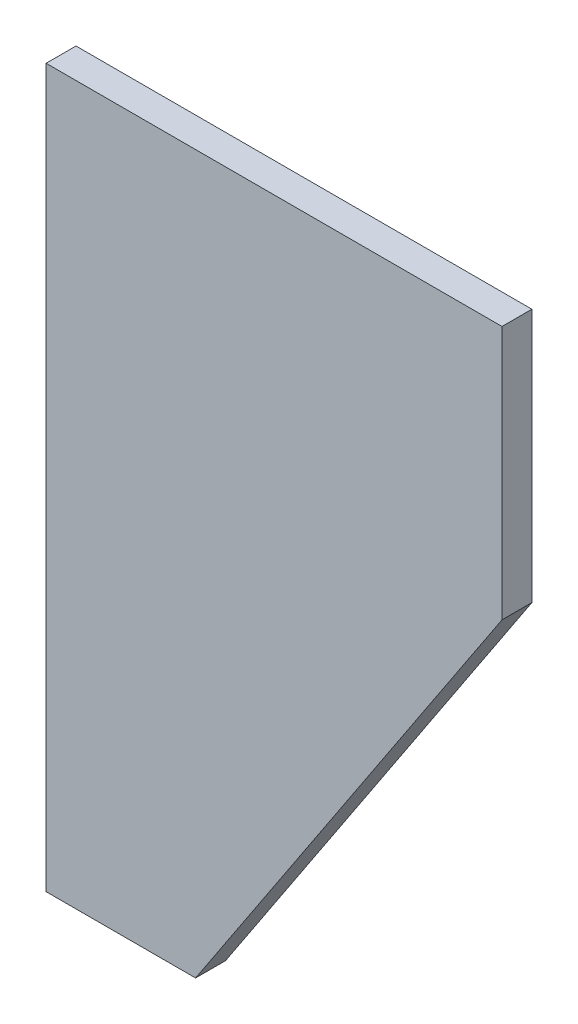
from build123d import *

# Parameters (mm, degrees)
EXTRUDE_1_DEPTH = 2


with BuildPart() as part:
    # 草图1 → 凸台-拉伸1 (new body)
    with BuildSketch(Plane.XY):
        Polygon((0, 0), (30.5, 0), (30.5, -17), (10, -48), (0, -48), align=None)
    extrude(amount=EXTRUDE_1_DEPTH)


solid = part.part
